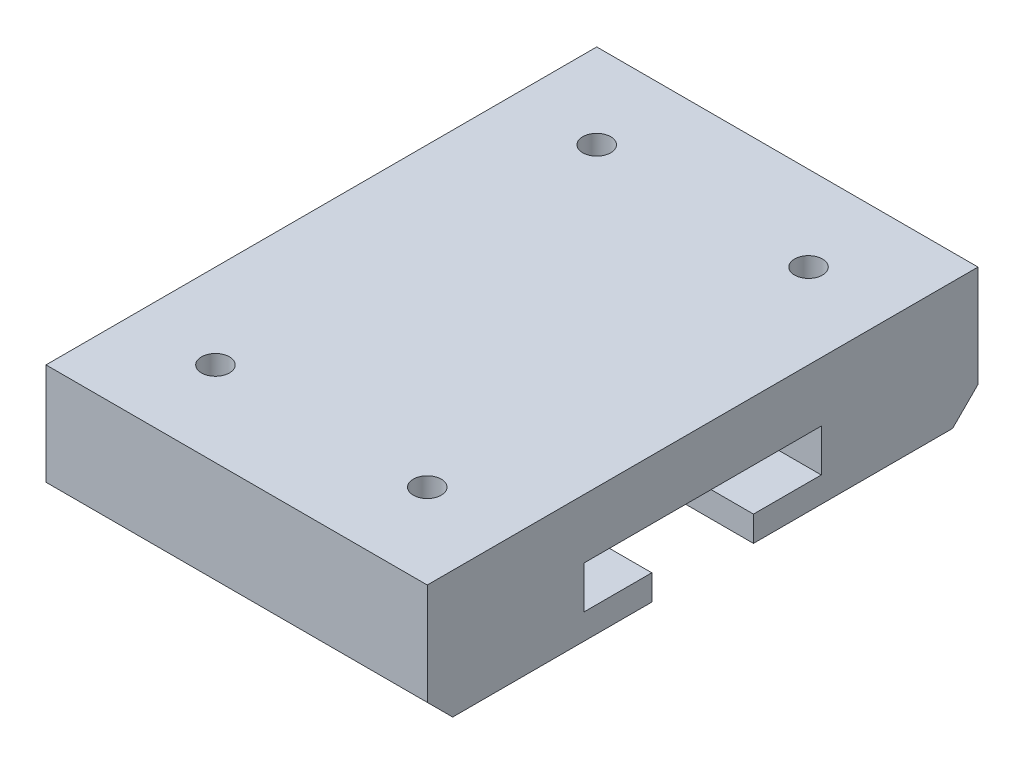
SolidWorks part; units mm, degrees
ref_plane "Front Plane" through (0, 0, 0) normal (0, 0, 1) x (1, 0, 0)
ref_plane "Top Plane" through (0, 0, 0) normal (0, 1, 0) x (1, 0, 0)
ref_plane "Right Plane" through (0, 0, 0) normal (1, 0, 0) x (0, 0, -1)
other "Configuration Table"
sketch "Sketch2" plane through (0, 0, 0) normal (1, 0, 0) x (0, 0, -1)
  line L0 (5, 0) -> (195, 0) construction
  line L1 (67.5, 0) -> (132.5, 0)
  line L2 (67.5, 0) -> (67.5, -15)
  line L3 (67.5, -15) -> (94, -15)
  line L4 (132.5, 0) -> (132.5, -15)
  line L5 (100, 0) -> (100, -29.5777) construction
  line L6 (94, -15) -> (94, -12)
  line L9 (106, -15) -> (132.5, -15)
  line L10 (94, -12) -> (86, -12)
  line L11 (86, -12) -> (86, -7)
  line L15 (86, -7) -> (114, -7)
  line L16 (114, -12) -> (114, -7)
  line L17 (106, -12) -> (114, -12)
  line L18 (106, -15) -> (106, -12)
  point P12 (100, 0)
  point P17 (100, -7)
  dimension "D1" = 15
  dimension "D2" = 65
  dimension "D3" = 3
  dimension "D4" = 8
  dimension "D5" = 5
  dimension "D6" = 14
extrude "Boss-Extrude1" add sketch "Sketch2" along normal mid plane 45
chamfer "Chamfer1" distance 3 angle 45 2 edges at (0, -15, -132.5) (0, -15, -67.5)
hole_wizard "M4 Tapped Hole1" positions "Sketch3" profile "Sketch4" tap size "M4" standard "GB" end condition through all
sketch "Sketch3" plane through (0, 0, 0) normal (0, 1, 0) x (1, 0, 0)
  point P0 (-12.5, 122.5)
  point P3 (12.5, 122.5)
  point P6 (-12.5, 77.5)
  point P9 (12.5, 77.5)
sketch "Sketch4" plane through (-12.5, 0, -122.5) normal (1, 0, 0) x (0, 0, 1)
  line L0 (0, 0) -> (0, 15)
  line L1 (0, 15) -> (1.65, 15)
  line L2 (1.65, 15) -> (1.65, 0)
  line L5 (1.65, 0) -> (0, 0)
  line L11 (0, -6.35) -> (0, 107.95) construction
  dimension "通孔螺纹孔钻头直径" = 3.3
  dimension "通孔螺纹孔钻头深度" = 15
cosmetic thread "Cosmetic Thread1" parameters "D2"=4
cosmetic thread "Cosmetic Thread2" parameters "D2"=4
cosmetic thread "Cosmetic Thread3" parameters "D2"=4
cosmetic thread "Cosmetic Thread4" parameters "D2"=4
